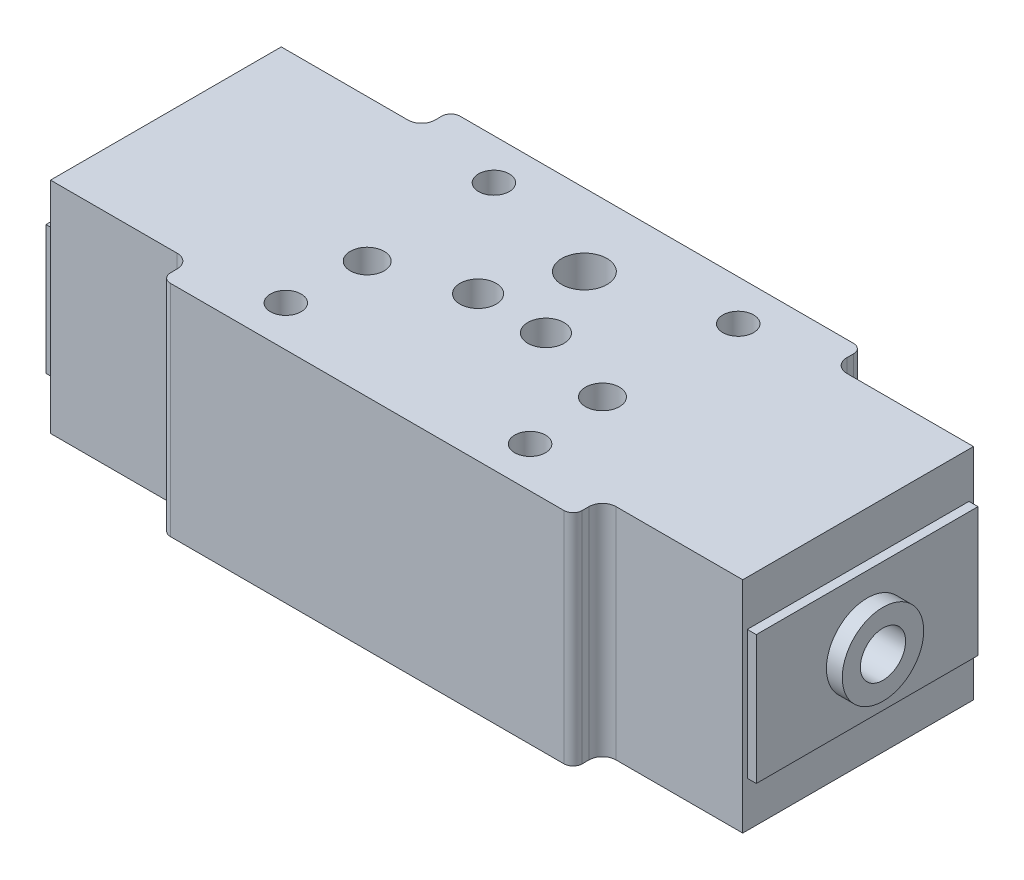
from build123d import *

# Parameters (mm, degrees)
BOSS_EXTRUDE_1_DEPTH = 24.25
SKETCH_2_W           = 49
SKETCH_2_H           = 28.5
SKETCH_2_R           = 3.024345666
BOSS_EXTRUDE_2_DEPTH = 2
SKETCH_3_R           = 9
BOSS_EXTRUDE_3_DEPTH = 5.5
SKETCH_4_R           = 3.4
SKETCH_4_R_2         = 5
SKETCH_4_R_3         = 4
SKETCH_4_R_4         = 3.75
CUT_EXTRUDE_1_DEPTH  = 101.5
SKETCH_5_R           = 5
CUT_EXTRUDE_2_DEPTH  = 169.843307537


with BuildPart() as part:
    # Sketch 1 → Boss-Extrude 1 (new, symmetric)
    with BuildSketch(Plane(origin=(0, 0, 0), x_dir=(1, 0, 0), z_dir=(0, 1, 0))):
        with BuildLine():
            Line((43.5, 32), (-43.5, 32))
            ThreePointArc((-43.5, 32), (-44.914213562, 31.414213562), (-45.5, 30))
            Line((-45.5, 30), (-45.5, 28.5))
            ThreePointArc((-45.5, 28.5), (-46.378679656, 26.378679656), (-48.5, 25.5))
            Line((-48.5, 25.5), (-76.5, 25.5))
            Line((-76.5, 25.5), (-76.5, -25.5))
            Line((-76.5, -25.5), (-48.5, -25.5))
            ThreePointArc((-48.5, -25.5), (-46.378679656, -26.378679656), (-45.5, -28.5))
            Line((-45.5, -28.5), (-45.5, -30))
            ThreePointArc((-45.5, -30), (-44.914213562, -31.414213562), (-43.5, -32))
            Line((-43.5, -32), (43.5, -32))
            ThreePointArc((43.5, -32), (44.914213562, -31.414213562), (45.5, -30))
            Line((45.5, -30), (45.5, -28.5))
            ThreePointArc((45.5, -28.5), (46.378679656, -26.378679656), (48.5, -25.5))
            Line((48.5, -25.5), (76.5, -25.5))
            Line((76.5, -25.5), (76.5, 25.5))
            Line((76.5, 25.5), (48.5, 25.5))
            ThreePointArc((48.5, 25.5), (46.378679656, 26.378679656), (45.5, 28.5))
            Line((45.5, 28.5), (45.5, 30))
            ThreePointArc((45.5, 30), (44.914213562, 31.414213562), (43.5, 32))
        make_face()
    extrude(amount=BOSS_EXTRUDE_1_DEPTH, both=True)

    # Sketch 2 → Boss-Extrude 2 (add)
    with BuildSketch(Plane(origin=(76.5, 0, 0), x_dir=(0, 0, -1), z_dir=(1, 0, 0))):
        Rectangle(SKETCH_2_W, SKETCH_2_H)
        Circle(SKETCH_2_R, mode=Mode.SUBTRACT)
    boss_extrude_2 = extrude(amount=BOSS_EXTRUDE_2_DEPTH)

    # Sketch 3 → Boss-Extrude 3 (add)
    with BuildSketch(Plane(origin=(76.5, 0, 0), x_dir=(0, 0, -1), z_dir=(1, 0, 0))):
        with Locations(Location((0, 0, 0), (0, 0, 180))):
            Circle(SKETCH_3_R)
    boss_extrude_3 = extrude(amount=BOSS_EXTRUDE_3_DEPTH)

    # Mirror 1: Boss-Extrude 2, Boss-Extrude 3 across plane
    add(boss_extrude_2.mirror(Plane(origin=(0, 0, 0), x_dir=(0, 0, 1), z_dir=(1, 0, 0))))
    add(boss_extrude_3.mirror(Plane(origin=(0, 0, 0), x_dir=(0, 0, 1), z_dir=(1, 0, 0))))

    # Sketch 4 → Cut-Extrude 1 (cut, through all)
    with BuildSketch(Plane(origin=(0, 24.25, 0), x_dir=(1, 0, 0), z_dir=(0, 1, 0))):
        with Locations(Location((-27, 23, 0), (0, 0, 270))):
            Circle(SKETCH_4_R)
        with Locations(Location((0, 16, 0), (0, 0, 270))):
            Circle(SKETCH_4_R_2)
        with Locations(Location((-7.5, 0, 0), (0, 0, 270))):
            Circle(SKETCH_4_R_3)
        with Locations(Location((-26, -6, 0), (0, 0, 270))):
            Circle(SKETCH_4_R_4)
        with Locations(Location((-27, -23, 0), (0, 0, 270))):
            Circle(SKETCH_4_R)
        with Locations(Location((7.5, 0, 0), (0, 0, 270))):
            Circle(SKETCH_4_R_3)
        with Locations(Location((27, -23, 0), (0, 0, 270))):
            Circle(SKETCH_4_R)
        with Locations(Location((26, -6, 0), (0, 0, 270))):
            Circle(SKETCH_4_R_4)
        with Locations(Location((27, 23, 0), (0, 0, 270))):
            Circle(SKETCH_4_R)
    extrude(amount=-CUT_EXTRUDE_1_DEPTH, mode=Mode.SUBTRACT)

    # Sketch 5 → Cut-Extrude 2 (cut, through all)
    with BuildSketch(Plane(origin=(82, 0, 0), x_dir=(0, 0, -1), z_dir=(1, 0, 0))):
        Circle(SKETCH_5_R)
    extrude(amount=-CUT_EXTRUDE_2_DEPTH, mode=Mode.SUBTRACT)


solid = part.part
